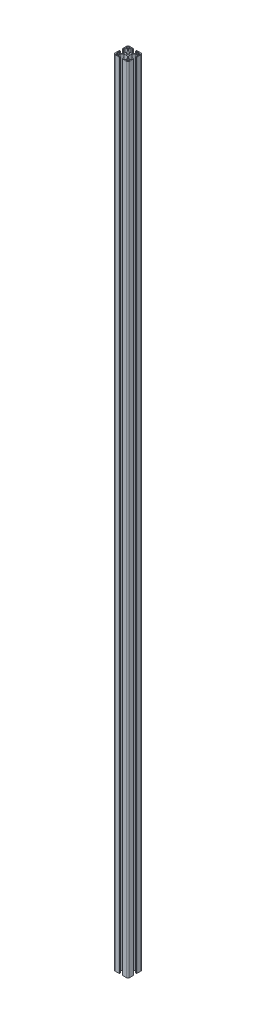
SolidWorks part; units mm, degrees
ref_plane "前视基准面" through (0, 0, 0) normal (0, 0, 1) x (1, 0, 0)
ref_plane "上视基准面" through (0, 0, 0) normal (0, 1, 0) x (1, 0, 0)
ref_plane "右视基准面" through (0, 0, 0) normal (1, 0, 0) x (0, 0, -1)
sketch "草图1" plane through (0, 0, 0) normal (0, 0, 1) x (1, 0, 0)
  line L0 (0, 0) -> (0, 2200)
  dimension "D1" = 2200
other "铝型材 40 X 40L X R4.5(1)"
ref_plane "基准面1" through (0, 0, 0) normal (0, 1, 0) x (-1, 0, 0)
sketch "Sketch1" plane through (0, 0, 0) normal (0, 1, 0) x (-1, 0, 0)
  line L0 (-5.1, 20) -> (-5.1, 19.5)
  line L1 (-5.1, 19.5) -> (-4.1, 19.5)
  line L2 (-4.1, 19.5) -> (-4.1, 17)
  line L3 (-6.1, 18.5) -> (-10.3, 18.5)
  line L4 (-15.5, -20) -> (-5.1, -20)
  line L5 (-20, -15.5) -> (-20, -5.1)
  line L6 (15.5, 20) -> (5.1, 20)
  line L7 (20, 15.5) -> (20, 5.1)
  line L8 (0, 14.8756) -> (0, 0) construction
  line L9 (0, 0) -> (14.1675, 0) construction
  line L10 (-10.3, 18.5) -> (-10.3, 11.3)
  line L11 (-10.3, 11.3) -> (-5, 6)
  line L12 (-5, 6) -> (5, 6)
  line L13 (10.3, 11.3) -> (5, 6)
  line L14 (10.3, 18.5) -> (10.3, 11.3)
  line L15 (6.1, 18.5) -> (10.3, 18.5)
  line L16 (4.1, 19.5) -> (4.1, 17)
  line L17 (5.1, 19.5) -> (4.1, 19.5)
  line L18 (5.1, 20) -> (5.1, 19.5)
  line L19 (-5.1, 20) -> (-15.5, 20)
  line L20 (20, 5.1) -> (19.5, 5.1)
  line L21 (11.8, 17.5) -> (15, 17.5)
  line L22 (11.8, 17.5) -> (11.8, 11.8)
  line L23 (11.8, 11.8) -> (17.5, 11.8)
  line L24 (17.5, 15) -> (17.5, 11.8)
  line L25 (19.5, 5.1) -> (19.5, 4.1)
  line L26 (19.5, 4.1) -> (17, 4.1)
  line L27 (17, 6.1) -> (17, 4.1)
  line L28 (18.5, 6.1) -> (17, 6.1)
  line L29 (18.5, 6.1) -> (18.5, 10.3)
  line L30 (18.5, 10.3) -> (11.3, 10.3)
  line L31 (11.3, 10.3) -> (6, 5)
  line L32 (6, 5) -> (6, -5)
  line L33 (11.3, -10.3) -> (6, -5)
  line L34 (18.5, -10.3) -> (11.3, -10.3)
  line L35 (18.5, -6.1) -> (18.5, -10.3)
  line L36 (18.5, -6.1) -> (17, -6.1)
  line L37 (17, -4.1) -> (17, -6.1)
  line L38 (19.5, -4.1) -> (17, -4.1)
  line L39 (19.5, -5.1) -> (19.5, -4.1)
  line L40 (20, -5.1) -> (19.5, -5.1)
  line L41 (5.1, -20) -> (5.1, -19.5)
  line L42 (5.1, -19.5) -> (4.1, -19.5)
  line L43 (4.1, -19.5) -> (4.1, -17)
  line L44 (6.1, -17) -> (4.1, -17)
  line L45 (6.1, -18.5) -> (6.1, -17)
  line L46 (6.1, -18.5) -> (10.3, -18.5)
  line L47 (10.3, -18.5) -> (10.3, -11.3)
  line L48 (10.3, -11.3) -> (5, -6)
  line L49 (5, -6) -> (-5, -6)
  line L50 (-10.3, -11.3) -> (-5, -6)
  line L51 (-10.3, -18.5) -> (-10.3, -11.3)
  line L52 (-6.1, -18.5) -> (-10.3, -18.5)
  line L53 (-6.1, -18.5) -> (-6.1, -17)
  line L54 (-4.1, -17) -> (-6.1, -17)
  line L55 (-4.1, -19.5) -> (-4.1, -17)
  line L56 (-5.1, -19.5) -> (-4.1, -19.5)
  line L57 (-5.1, -20) -> (-5.1, -19.5)
  line L58 (-20, -5.1) -> (-19.5, -5.1)
  line L59 (5.1, -20) -> (15.5, -20)
  line L60 (-20, 5.1) -> (-20, 15.5)
  line L61 (-19.5, -5.1) -> (-19.5, -4.1)
  line L62 (-6.1, 18.5) -> (-6.1, 17)
  line L63 (-6.1, 17) -> (-4.1, 17)
  line L64 (6.1, 18.5) -> (6.1, 17)
  line L65 (4.1, 17) -> (6.1, 17)
  line L66 (-19.5, -4.1) -> (-17, -4.1)
  line L67 (-15, 17.5) -> (-11.8, 17.5)
  line L68 (-17.5, 15) -> (-17.5, 11.8)
  line L69 (-17.5, 11.8) -> (-11.8, 11.8)
  line L70 (-11.8, 17.5) -> (-11.8, 11.8)
  line L71 (-17, -6.1) -> (-17, -4.1)
  line L72 (-18.5, -6.1) -> (-17, -6.1)
  line L73 (-18.5, -6.1) -> (-18.5, -10.3)
  line L74 (-18.5, -10.3) -> (-11.3, -10.3)
  line L75 (-11.3, -10.3) -> (-6, -5)
  line L76 (-6, -5) -> (-6, 5)
  line L77 (-11.3, 10.3) -> (-6, 5)
  line L78 (-18.5, 10.3) -> (-11.3, 10.3)
  line L79 (-18.5, 6.1) -> (-18.5, 10.3)
  line L80 (-18.5, 6.1) -> (-17, 6.1)
  line L81 (-17, 4.1) -> (-17, 6.1)
  line L82 (-19.5, 4.1) -> (-17, 4.1)
  line L83 (-19.5, 5.1) -> (-19.5, 4.1)
  line L84 (-20, 5.1) -> (-19.5, 5.1)
  line L85 (20, -5.1) -> (20, -15.5)
  line L87 (-17.5, -11.8) -> (-11.8, -11.8)
  line L88 (-17.5, -11.8) -> (-17.5, -15)
  line L89 (-15, -17.5) -> (-11.8, -17.5)
  line L90 (-11.8, -11.8) -> (-11.8, -17.5)
  line L91 (11.8, -11.8) -> (17.5, -11.8)
  line L92 (11.8, -11.8) -> (11.8, -17.5)
  line L93 (11.8, -17.5) -> (15, -17.5)
  line L94 (17.5, -11.8) -> (17.5, -15)
  circle A0 centre (0, 0) radius 3.4
  arc A1 (-20, 15.5) -> (-15.5, 20) centre (-15.5, 15.5) cw
  arc A2 (20, 15.5) -> (15.5, 20) centre (15.5, 15.5) ccw
  arc A3 (-15.5, -20) -> (-20, -15.5) centre (-15.5, -15.5) cw
  arc A4 (15.5, -20) -> (20, -15.5) centre (15.5, -15.5) ccw
  arc A5 (-15, 17.5) -> (-17.5, 15) centre (-15, 15) ccw
  arc A6 (17.5, 15) -> (15, 17.5) centre (15, 15) ccw
  arc A7 (17.5, -15) -> (15, -17.5) centre (15, -15) cw
  arc A8 (-17.5, -15) -> (-15, -17.5) centre (-15, -15) ccw
  point P2 (0, 10)
  point P4 (0, 0)
  point P5 (-20, -20)
  point P6 (20, -20)
  point P7 (20, 20)
  point P8 (-20, 20)
  point P36 (-20, 20)
  point P39 (20, 20)
  point P121 (0, 0)
  dimension "D1" = 20.6
  dimension "D2" = 40
  dimension "D3" = 8.2
  dimension "D4" = 10.2
  dimension "D5" = 14
  dimension "D6" = 6.8
  dimension "D7" = 4.5
  dimension "D8" = 45
  dimension "D12" = 2.5
  dimension "D13" = 5.7
  dimension "D14" = 1.5
  dimension "D18" = 2.5
  dimension "D19" = 2.5
  dimension "D15" = 2.5
  dimension "D9" = 0.5
  dimension "D10" = 1.5
  dimension "D11" = 10
  dimension "D16" = 3
  dimension "D17" = 2
  dimension "D20" = 1.5
  dimension "D21" = 2.5
